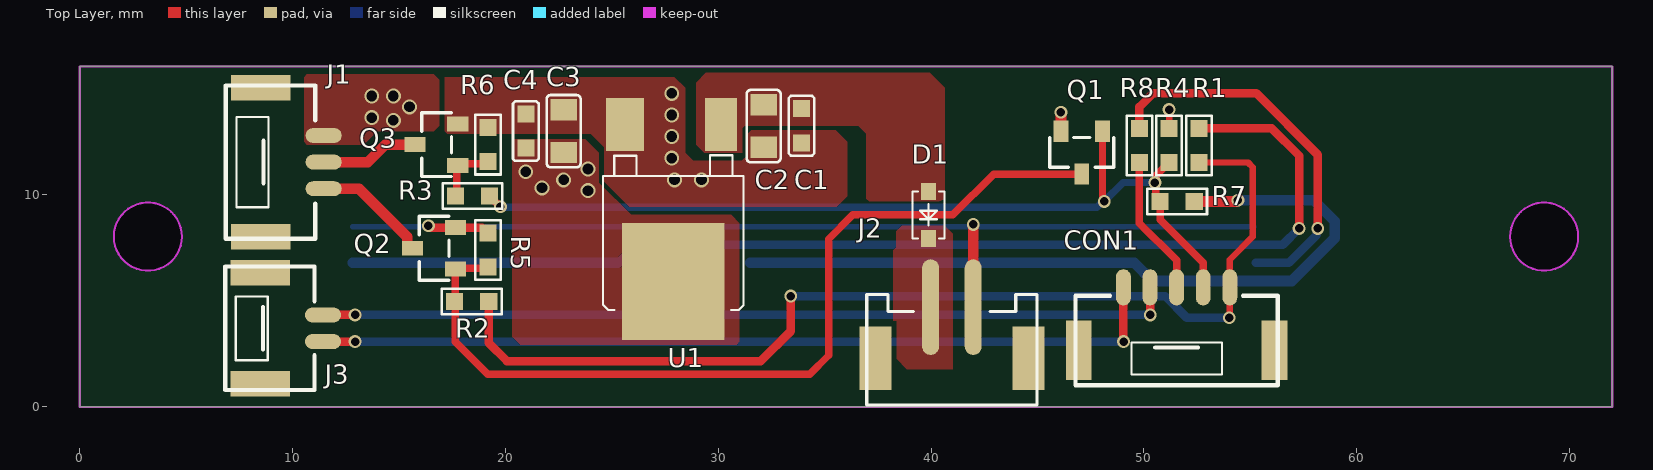
[diagram p0: Top Layer view]
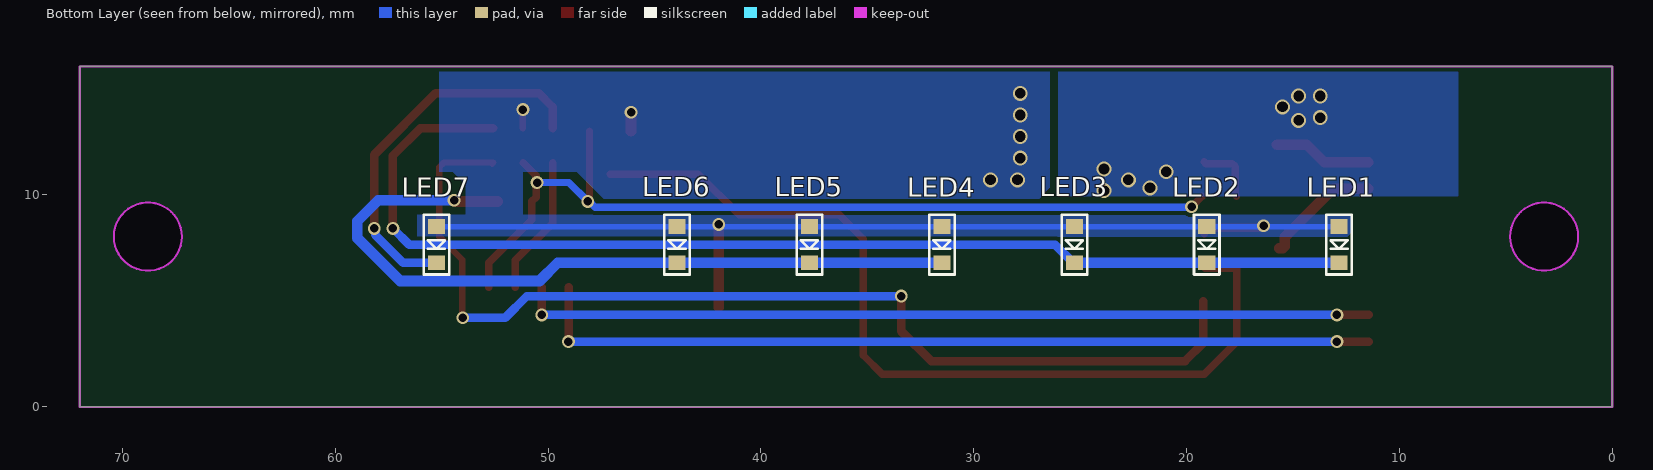
[diagram p1: Bottom Layer view, seen from below]
# Altium PCB MISC88840.PcbDoc
Units mm, origin at the board's own origin, x right, y up, seen from the top; angles counter-clockwise.
Board outline 72 x 16 mm, 2 copper layers (Top Layer, Bottom Layer); 28 components, 16 nets, 72 pads, 32 vias.

## Layer stack, top to bottom (the 12.6 mil dielectric is the usual default, probably not edited)
Top Solder: solder mask 0.0102, Solder Resist, Dk 3.5
Top Layer: signal copper 0.0356
Dielectric 1: dielectric 0.32, FR-4, Dk 4.8
Bottom Layer: signal copper 0.0356
Bottom Solder: solder mask 0.0102, Solder Resist, Dk 3.5

## Board outline
0,0 72,0 72,16 0,16
cut-out: 3.2,6.4 cw(c3.2,8) 1.6,8 cw(c3.2,8) 3.2,9.6 cw(c3.2,8) 4.8,8 cw(c3.2,8)
cut-out: 67.2,8 ccw(c68.8,8) 68.8,6.4 ccw(c68.8,8) 70.4,8 ccw(c68.8,8) 68.8,9.6 ccw(c68.8,8)

## Design rules (kind name [scope] priority, off if disabled: settings)
Clearance [All] p1: gap=0.2 ignorepadtopadclearanceinfootprint=TRUE
PolygonConnect [All] p1: connectstyle=Direct reliefconductorwidth=0.254 reliefentries=4 polygonreliefangle="90 Angle" airgapwidth=0.254
RoutingVias [All] p1: holewidth=0.711 width=1.27 viastyle="Through Hole" minholewidth=0.711 minwidth=1.27 maxholewidth=0.711 maxwidth=1.27
SilkToSilkClearance [All] p1: silktosilkclearance=0.01
SilkToSolderMaskClearance [IsPad] p1: minsilkscreentomaskgap=0 clearancetoexposedcopper=TRUE
SolderMaskExpansion [All] p1: expansion=0.102 istentingtop=FALSE
SupplyNets "Schematic Supply Nets_1" [InNet('VCC5V')] p1: voltage=0.000
SupplyNets "Schematic Supply Nets" [InNet('B-')] p2: voltage=0.000
Width [All] p1: maxlimit=100 minlimit=0.254 preferedwidth=0.254
28 further rules are at their usual default settings.

## Components (designator, comment, footprint, x,y, rotation, side; value= is the part's Value field where it differs from the comment)
C1 "100nF/50V" C0603A 33.909,13.208 r90 top
C2 "10uF/25V" C0805A 32.131,13.192 r90 top
C3 "10uF/25V" C0805A 22.733,12.954 r270 top
C4 "100nF/50V" C0603A 20.955,12.954 r270 top
CON1 "5PIN ribbon cable" GH1.25-5PIN立贴带扣耐温260℃ 51.534,5.617 r0 top
D1 "SS34/SMA" SOD323 39.878,9.017 r90 top
J1 "3PIN 1.25" GH1.25-3PIN立贴带扣耐温260℃ 11.459,11.501 r270 top
J2 "2PIN" "HY2.0WT-2A/P 立贴带扣耐温260℃" 40.977,4.686 r0 top
J3 "2PIN" GH1.25-2PIN立贴带扣耐温260℃ 11.43,3.693 r270 top
LED1 "" LED0603A 12.827,7.62 r90 bottom
LED2 "" LED0603A 19.05,7.62 r90 bottom
LED3 "" LED0603A 25.273,7.62 r90 bottom
LED4 "" LED0603A 31.496,7.62 r90 bottom
LED5 "" LED0603A 37.719,7.62 r90 bottom
LED6 "" LED0603A 43.942,7.62 r90 bottom
LED7 "" LED0603A 55.245,7.62 r90 bottom
Q1 "CJ2300/SOT23" SOT23-3 47.076,11.954 r180 top
Q2 "CJ2300/SOT23" SOT23-3 16.653,7.452 r90 top
Q3 "CJ2300/SOT23" SOT23-3 16.764,12.319 r90 top
R1 "1K/5%" R0603A 52.578,12.281 r90 top
R2 "100K/5%" R0603A 18.415,4.953 r180 top
R3 "100K/5%" R0603A 18.453,9.906 r180 top
R4 "100K/5%" R0603A 51.181,12.281 r90 top
R5 "100K/5%" R0603A 19.177,7.366 r270 top
R6 "100K/5%" R0603A 19.177,12.319 r270 top
R7 "1K/5%" R0603A 51.562,9.652 r0 top
R8 "1K/5%" R0603A 49.784,12.281 r270 top
U1 "78M05/TO252" TO-252-A 30.099,13.081 r180 top

## Footprints (in the part's own frame and the unit in brackets; to place one, negate y for a bottom-side part, rotate by r counter-clockwise, add the part's x,y. Pads: shape width x height; smd on the part's side, far side on the other; paste and mask are expansions set on the pad)
C0603A [mm] "贴片电容"
  rect 0.8x0.8 smd mask+0.08: 1(-0.8,0) 2(0.8,0)
  silkscreen extent -1.4,-0.6 1.4,0.6
C0805A [mm] "贴片电容"
  rect 1x1.25 smd: 1(-1,0)
  rect 1x1.25 smd mask+0.102: 2(1,0)
  silkscreen extent -1.7,-0.8 1.7,0.8
GH1.25-2PIN立贴带扣耐温260℃ [mm] "立贴带扣耐温260℃"
  rect 1.2x2.8 smd: 0(-2.6,-2.95) 0(2.6,-2.95)
  oval 0.7x1.7 smd: 1(-0.625,0) 2(0.625,0)
  silkscreen extent -2.9,-4.6 2.9,-0.4
GH1.25-3PIN立贴带扣耐温260℃ [mm] "立贴带扣耐温260℃"
  rect 1.2x2.8 smd: 0(-3.5,-2.95) 0(3.5,-2.95)
  oval 0.7x1.7 smd: 1(-1.25,0) 2(0,0) 3(1.25,0)
  silkscreen extent -3.6,-4.6 3.6,-0.4
GH1.25-5PIN立贴带扣耐温260℃ [mm] "立贴带扣耐温260℃"
  rect 1.2x2.8 smd: 0(-4.6,-2.95) 0(4.6,-2.95)
  oval 0.7x1.7 smd: 1(-2.5,0) 2(-1.25,0) 3(0,0) 4(1.25,0) 5(2.5,0)
  silkscreen extent -4.75,-4.6 4.75,-0.4
"HY2.0WT-2A/P 立贴带扣耐温260℃" [mm] "卧贴连接器"
  rect 1.5x3 smd: 0(-3.6,-2.4) 0(3.6,-2.4)
  oval 0.8x4.5 smd: 1(-1,0) 2(1,0)
  silkscreen extent -4,-4.6 4,0.6
LED0603A [mm] "贴片LED"
  rect 0.7x0.8 smd: 1(-0.85,0) 2(0.85,0)
  silkscreen extent -1.4,-0.6 1.4,0.6
R0603A [mm] "贴片电阻"
  rect 0.8x0.8 smd mask+0.08: 1(-0.8,0) 2(0.8,0)
  silkscreen extent -1.4,-0.6 1.4,0.6
SOD323 [mm] "贴片二极管"
  rect 0.8x0.7 smd: 1(-1.1,0) 2(1.1,0)
  silkscreen extent -1.1,-0.75 1.1,0.75
SOT23-3 [mm] "贴片IC/MOS*"
  rect 0.7x1 smd: 1(-0.975,-1) 2(0.975,-1) 3(0,1.016)
  silkscreen extent -1.5,-0.7 1.5,0.7
TO-252-A [mm]
  rect 1.5x2.5 smd: 1(-0.026,-0.189)
  rect 1.8x2.5 smd: 2(4.484,-0.189)
  rect 4.8x5.5 smd: 3(2.214,7.181)
  silkscreen extent -1.09,1.26 5.51,8.53, body extent -0.95,-0.35 5.35,9.65, height 2.5

## Part data
C1 C4: library part C0603, "SMD capacitor"
C2 C3: library part C0805, "SMD capacitor"
CON1: library part 5PIN, "10PIN dual row"
D1: library part T4, "Fast recovery diode"
J1: library part 3PIN, "DC socket 3PIN, 2.0 pitch"
J2 J3: "DC socket right angle 90°, 2.0 pitch"
LED1 LED2 LED3 LED4 LED5 LED6 LED7: library part "LED 白发蓝", "SMD LED"
Q1 Q2 Q3: library part MOS-N, "Single N-channel MOSFET"
R1 R2 R3 R4 R5 R6 R7 R8: library part Res0603, "SMD resistor"
U1: library part HT7533_SO89, "SMD LDO"

## Via types
v1: diameter 0.6, hole 0.4, Top Layer to Bottom Layer, tented both sides, 16 vias
v2: diameter 0.7, hole 0.5, Top Layer to Bottom Layer, tented both sides, 16 vias

## Nets (pads, with @x,y where several pads share a name; then routed paths per layer and width w, separated by ;. In a path a pad name is that pad's centre, name@x,y a point inside that pad or via, vN(x,y) a via of type N, cw(c..) or ccw(c..) an arc to the next point about the centre after c; other vN are vias at no path point)
B-: CON1.1 J3.2 | length 40.2
  Top Layer w0.4: J3.2 v1(12.934,3.068) ; CON1.1 49.038,5.613 49.038,3.072 v1(49.042,3.068)
  Bottom Layer w0.4: v1(12.934,3.068) v1(49.042,3.068)
DS-: C1.1 C2.1 C3.1 C4.1 J2.2 LED1.2 LED2.2 LED3.2 LED4.2 LED5.2 LED6.2 LED7.2 Q1.2 Q2.2 Q3.2 R4.2 R5.1 R6.1 U1.2 | length 50.9
  Top Layer w0.3: R4.2 v1(51.181,13.97)
  Top Layer w0.4: v1(16.383,8.509) 16.437,8.509 16.519,8.427 Q2.2 18.916,8.427 R5.1
  Top Layer w0.5: J2.2 v1(41.977,8.569) ; Q1.2 v1(46.101,13.84)
  Bottom Layer w0.254: LED1.2 LED2.2 LED3.2 LED4.2 LED5.2 LED6.2 LED7.2@55.165,8.47
  other v2: 27.94,10.668 29.21,10.668 27.813,11.684 27.813,12.7 27.813,13.716 27.813,14.732
KEY: CON1.2 J3.1 | length 40.2
  Top Layer w0.4: J3.1 v1(12.934,4.318) ; CON1.2 50.288,5.613 50.288,4.322 v1(50.292,4.318)
  Bottom Layer w0.4: v1(12.934,4.318) v1(50.292,4.318)
LED1: CON1.5 R1.1 R2.1 | length 49.9
  Top Layer w0.3: R1.1 52.629,11.43 52.68,11.481 54.891,11.481 55.118,11.254 55.118,8.001 54.034,6.917 CON1.5 54.022,5.605 54.022,4.203 v1(54.01,4.191)
  Top Layer w0.4: R2.1 19.215,3.004 20.066,2.153 31.998,2.153 33.401,3.556 v1(33.401,5.207)
  Bottom Layer w0.4: v1(33.401,5.207) 50.99,5.207 52.006,4.191 v1(54.01,4.191)
LED2: CON1.4 Q1.1 R3.1 R4.1 R7.1 | length 42.4
  Top Layer w0.35: R3.1 v1(19.761,9.398) ; Q1.1 48.051,9.802 48.133,9.72 v1(48.133,9.652) ; v1@50.419,10.541 50.445,10.541 50.561,10.426 50.561,9.853 R7.1 50.762,8.801 52.784,6.779 CON1.4 ; v1(50.513,10.541) 50.561,10.589 50.561,10.861 R4.1@51.162,11.462
  Bottom Layer w0.35: v1(19.761,9.398) 19.778,9.381 47.794,9.381 48.065,9.652 v1(48.133,9.652) 49.022,10.541 v1(50.513,10.541)
LED3: CON1.3 R8.2 | length 6.6
  Top Layer w0.35: R8.2 49.784,8.636 51.534,6.886 CON1.3
LED_B: J1.3 Q2.3 | length 5.6
  Top Layer w0.5: J1.3 13.117,10.251 15.387,7.981 15.387,7.552 15.487,7.452 Q2.3
LED_G: J1.2 Q3.3 | length 4.6
  Top Layer w0.5: J1.2 13.533,11.501 14.351,12.319 Q3.3
NetC1_2: C1.2 C2.2 D1.2 U1.1
NetLED1_1: LED1.1 LED2.1 LED3.1 R1.2 | length 53.8
  Top Layer w0.4: R1.2 56.007,13.081 57.285,11.803 v1(57.285,8.382)
  Bottom Layer w0.4: LED3.1 25.323,6.77 26.173,7.62 56.523,7.62 v1(57.285,8.382)
  Bottom Layer w0.5: LED1.1 LED2.1 LED3.1
NetLED4_1: LED4.1 LED5.1 LED6.1 R7.2 | length 36.5
  Top Layer w0.5: R7.2 54.329,9.652 54.387,9.71 v1(54.414,9.71)
  Bottom Layer w0.5: LED4.1 LED5.1 49.546,6.77 50.4,5.916 56.95,5.916 58.97,7.936 58.97,8.715 57.975,9.71 v1(54.414,9.71)
NetLED7_1: LED7.1 R8.1 | length 18.1
  Top Layer w0.4: R8.1 49.784,14.097 50.419,14.732 55.281,14.732 58.166,11.847 v1(58.166,8.382)
  Bottom Layer w0.4: LED7.1 56.808,6.77 58.128,8.09 58.128,8.344 v1(58.166,8.382)
NetQ1_3: Q1.3 Q2.1 R2.2 R5.2 | length 42.2
  Top Layer w0.35: R5.2 19.133,6.522 17.698,6.522 Q2.1 17.634,6.458 17.634,3.067 19.177,1.524 34.29,1.524 35.179,2.413 35.179,7.874 36.322,9.017 41.021,9.017 42.942,10.938 Q1.3
NetQ3_1: Q3.1 R3.2 R6.2 | length 3
  Top Layer w0.35: R3.2 17.709,9.962 17.709,11.289 Q3.1 17.851,11.431 19.089,11.431 R6.2
P+: D1.1 J2.1
VCC5V: C3.2 C4.2 J1.1 U1.3
  other v2: 23.876,10.16 21.717,10.287 22.733,10.668 20.955,11.049 23.876,11.176 14.732,13.462 13.716,13.589 15.494,14.097 13.716,14.605 14.732,14.605
pads on no net: CON1.0 J1.0 J2.0 J3.0

## Polygon pours and split planes (outlines as drawn)
DS- on Top Layer "DS-_L01_P006" (solid, pour order 6): 31.374,12.822 31.369,12.827 31.623,13.081 35.433,13.081 36.068,12.446 36.068,9.906 35.56,9.398 25.781,9.398 24.638,10.541 24.638,12.192 24.003,12.827 17.272,12.827 17.145,12.954 17.145,15.494 27.94,15.494 28.448,14.986 28.448,11.938 28.829,11.557 31.1,11.557 31.374,11.831
VCC5V on Top Layer "VCC5V_L01_P003" (solid, pour order 3): 10.541,15.494 10.668,15.621 16.637,15.621 16.891,15.367 16.891,13.208 16.637,12.954 13.97,12.954 13.335,12.319 10.668,12.319 10.541,12.446
VCC5V on Top Layer "VCC5V_L01_P002" (solid, pour order 2): 30.988,8.636 30.607,9.017 25.908,9.017 24.384,10.541 24.384,11.938 23.749,12.573 20.32,12.573 20.32,3.302 20.701,2.921 30.861,2.921 30.988,3.048
NetC1_2 on Top Layer "NETC1_2_L01_P001" (solid, pour order 1): 31.115,11.938 29.337,11.938 28.956,12.319 28.956,15.24 29.718,16.002 39.624,16.002 40.64,14.986 40.64,9.652 40.513,9.525 40.386,9.652 37.084,9.652 36.957,9.779 36.957,12.827 36.576,13.208 31.242,13.208 31.115,13.081
P+ on Top Layer "P+_L01_P000" (solid, remove dead copper, pour order 0): 38.227,7.366 38.354,7.493 38.354,8.255 38.608,8.509 40.64,8.509 41.021,8.128 41.021,1.778 38.862,1.778 38.1,2.54 38.227,2.667 38.227,3.175
DS- on Bottom Layer "DS-_L02_P007" (solid, pour order 7): 47.371,9.779 48.641,11.049 51.181,11.049 51.181,8.89 53.721,8.89 53.86,9.029 53.86,10.426 54.483,11.049 55.118,11.049 55.118,16 26.416,16 26.416,10.287 26.924,9.779
VCC5V on Bottom Layer "VCC5V_L02_P005" (solid, remove dead copper, pour order 5): 7.239,9.906 7.239,15.875 7.364,16 26.035,16 26.035,9.906
DS- on Bottom Layer "DS-_L02_P004" (solid, pour order 4): 56.134,8.001 56.134,9.017 12.192,9.017 12.192,8.255 12.446,8.001

## Keep-outs
Keep-Out Layer:
  circle w0.1: c68.8,8 r1.6
  circle w0.1: c3.2,8 r1.6
  lines w0.1: 0,0 0,16 72,16 72,0 0,0

## Silkscreen, mask and mechanical layers (free items; w line width, h text height)
Mechanical 1:
  lines w0.1: 6.3,0 6.3,15.976